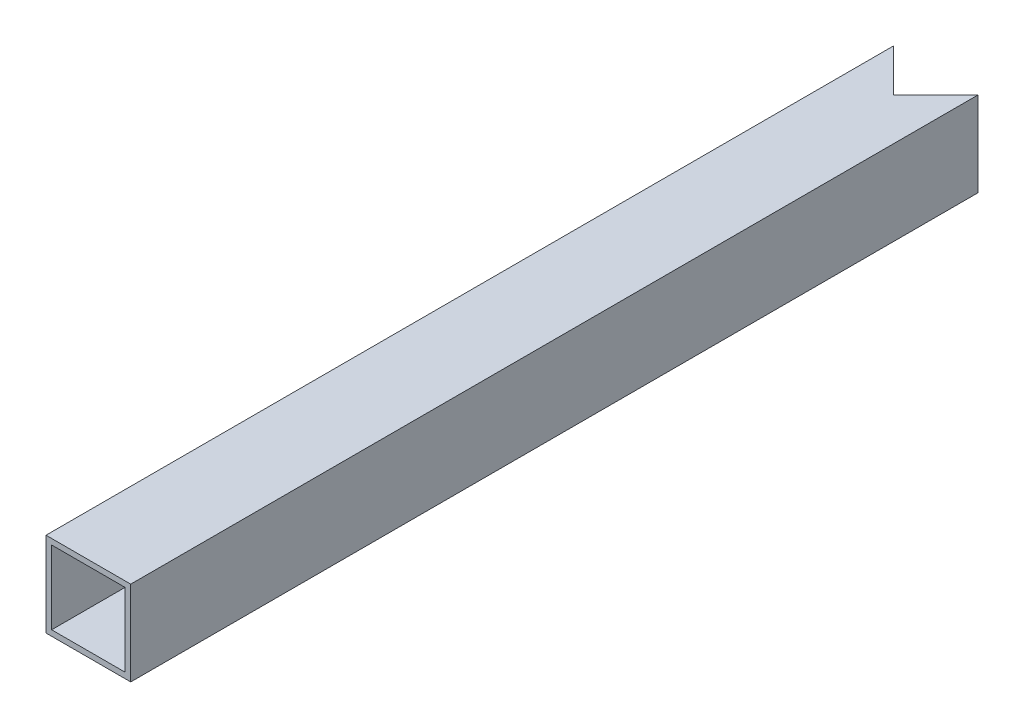
from build123d import *

# Parameters (mm, degrees)
SKETCH_1_W          = 30
SKETCH_1_H          = 30
SKETCH_1_W_2        = 26
SKETCH_1_H_2        = 26
EXTRUDE_1_DEPTH     = 150
CUT_EXTRUDE_1_DEPTH = 102


with BuildPart() as part:
    # 草图1 → 凸台-拉伸1 (new, symmetric)
    with BuildSketch(Plane.XY):
        Rectangle(SKETCH_1_W, SKETCH_1_H)
        Rectangle(SKETCH_1_W_2, SKETCH_1_H_2, mode=Mode.SUBTRACT)
    extrude(amount=EXTRUDE_1_DEPTH, both=True)

    # 草图3 → 切除-拉伸1 (cut)
    with BuildSketch(Plane(origin=(0, 15, 0), x_dir=(1, 0, 0), z_dir=(0, 1, 0))):
        Polygon((-15, 150), (0, 135), (15, 150), align=None)
    extrude(amount=-CUT_EXTRUDE_1_DEPTH, mode=Mode.SUBTRACT)


solid = part.part
